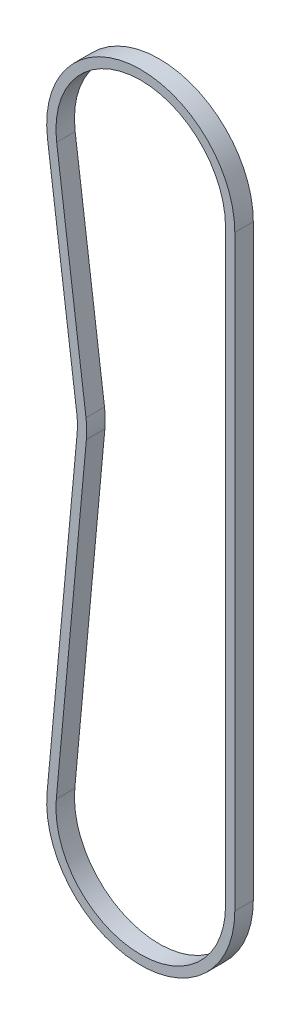
from build123d import *

# Parameters (mm, degrees)
EXTRUDE_1_DEPTH = 10


with BuildPart() as part:
    # 草图2 → 拉伸-薄壁1 (new, symmetric)
    with BuildSketch(Plane.XY):
        with BuildLine():
            Line((101.625, -635), (101.625, -1e-09))
            ThreePointArc((101.625, -2e-09), (-6.6169457, 101.409351915), (-100.763322845, -13.205809105))
            Line((-100.763322845, -13.205809104), (-69.067097403, -255.055208275))
            ThreePointArc((-69.067097403, -255.055208275), (-68.39008171, -264.093056524), (-68.7192023, -273.15024874))
            Line((-68.7192023, -273.15024874), (-101.19646024, -625.677068065))
            ThreePointArc((-101.19646024, -625.677068065), (-4.666387955, -736.517808529), (101.625, -635))
        make_face()
        with BuildLine():
            Line((91.625, -635), (91.625, -1e-09))
            ThreePointArc((91.625, -1e-09), (-5.965831732, 91.430571899), (-90.848112725, -11.906344494))
            Line((-90.848112725, -11.906344494), (-59.151887283, -253.755743665))
            ThreePointArc((-59.151887283, -253.755743665), (-58.391929391, -263.900832127), (-58.761371034, -274.067634416))
            Line((-58.761371034, -274.067634416), (-91.238628974, -626.594453741))
            ThreePointArc((-91.238628974, -626.594453741), (-4.207210789, -726.528356275), (91.625, -635))
        make_face(mode=Mode.SUBTRACT)
    extrude(amount=EXTRUDE_1_DEPTH, both=True)


solid = part.part
